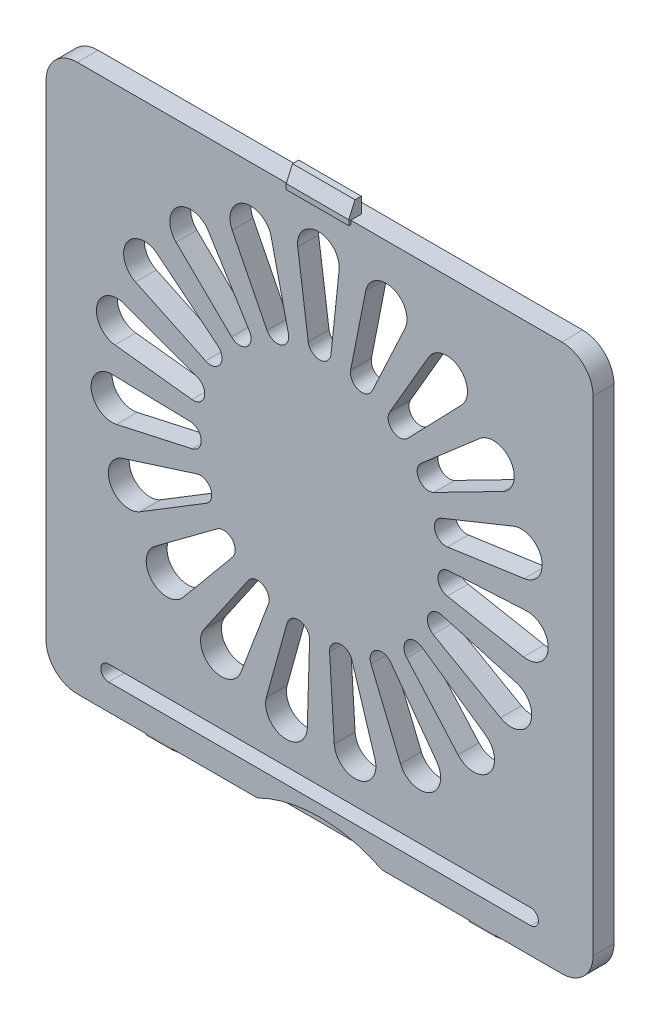
SolidWorks part; units mm, degrees
ref_plane "Front Plane" through (0, 0, 0) normal (0, 0, 1) x (1, 0, 0)
ref_plane "Top Plane" through (0, 0, 0) normal (0, 1, 0) x (1, 0, 0)
ref_plane "Right Plane" through (0, 0, 0) normal (1, 0, 0) x (0, 0, -1)
other "Configuration Table"
sketch "Sketch1" plane through (0, 0, 0) normal (0, 0, 1) x (1, 0, 0)
  line L1 (-23.25, 26.25) -> (23.25, 26.25)
  line L2 (-26.25, 23.25) -> (-26.25, -23.25)
  line L3 (-23.25, -26.25) -> (23.25, -26.25)
  line L4 (26.25, 23.25) -> (26.25, -23.25)
  line L5 (-26.25, 26.25) -> (26.25, -26.25) construction
  line L6 (-26.25, -26.25) -> (26.25, 26.25) construction
  line L11 (-20, -20) -> (20, 20) construction
  line L12 (-20, 20) -> (20, -20) construction
  arc A4 (23.25, -26.25) -> (26.25, -23.25) centre (23.25, -23.25) ccw
  arc A5 (-26.25, -23.25) -> (-23.25, -26.25) centre (-23.25, -23.25) ccw
  arc A6 (-23.25, 26.25) -> (-26.25, 23.25) centre (-23.25, 23.25) ccw
  arc A7 (23.25, 26.25) -> (26.25, 23.25) centre (23.25, 23.25) cw
  point P0 (0, 0)
  point P6 (0, 0)
  dimension "D6" = 3
  dimension "D1" = 52.5
  dimension "D2" = 52.5
extrude "Boss-Extrude1" add sketch "Sketch1" along normal blind 2
sketch "Sketch2" plane through (0, 0, 2) normal (0, 0, 1) x (1, 0, 0)
  line L6 (-20.25, -23) -> (20.25, -23) construction
  line L7 (-20.25, -22.25) -> (20.25, -22.25)
  line L8 (-20.25, -23.75) -> (20.25, -23.75)
  line L9 (26.25, -23.25) -> (26.25, 23.25) construction
  line L10 (-26.25, 23.25) -> (-26.25, -23.25) construction
  line L11 (-23.25, -26.25) -> (23.25, -26.25) construction
  line L12 (-2.0944, 21.4802) -> (-1.0899, 14.1016)
  line L13 (1.8762, 21.5399) -> (1.0939, 14.1344)
  line L14 (23.25, 26.25) -> (-23.25, 26.25) construction
  line L15 (4.4254, 21.0912) -> (2.9797, 13.7863)
  line L16 (8.2003, 19.8584) -> (5.0559, 13.1082)
  line L17 (10.4657, 18.6063) -> (6.7264, 12.1666)
  line L18 (13.6358, 16.2146) -> (8.4699, 10.8512)
  line L19 (15.3719, 14.2948) -> (9.7442, 9.4182)
  line L20 (17.5936, 11.0033) -> (10.9662, 7.6079)
  line L21 (18.6123, 8.6238) -> (11.7061, 5.8387)
  line L22 (19.6449, 4.7893) -> (12.274, 3.7298)
  line L23 (19.8358, 2.208) -> (12.3994, 1.8162)
  line L24 (19.5674, -1.754) -> (12.2518, -0.3629)
  line L25 (18.9097, -4.2575) -> (11.7491, -2.2134)
  line L26 (17.3694, -7.9177) -> (10.9019, -4.2265)
  line L27 (15.9345, -10.072) -> (9.8256, -5.8136)
  line L28 (13.2892, -13.0337) -> (8.3706, -7.4426)
  line L29 (11.2326, -14.6054) -> (6.8373, -8.5942)
  line L30 (7.7689, -16.5477) -> (4.9323, -9.6624)
  line L31 (5.3134, -17.3664) -> (3.1081, -10.2538)
  line L32 (1.4067, -18.0788) -> (0.9594, -10.6456)
  line L33 (-1.1816, -18.0559) -> (-0.9579, -10.6126)
  line L34 (-5.1079, -17.4612) -> (-3.1174, -10.2855)
  line L35 (-7.5485, -16.5991) -> (-4.9201, -9.6317)
  line L36 (-11.069, -14.7617) -> (-6.8564, -8.6211)
  line L37 (-13.0975, -13.1538) -> (-8.3492, -7.4174)
  line L38 (-15.8306, -10.273) -> (-9.8524, -5.8329)
  line L39 (-17.2271, -8.0936) -> (-10.8735, -4.2097)
  line L40 (-18.8767, -4.4813) -> (-11.7808, -2.223)
  line L41 (-19.4899, -1.9666) -> (-12.2194, -0.3562)
  line L42 (-19.8772, 1.9856) -> (-12.4325, 1.8175)
  line L43 (-19.6406, 4.5631) -> (-12.2412, 3.7255)
  line L44 (-18.7237, 8.4269) -> (-11.7369, 5.8506)
  line L45 (-17.663, 10.788) -> (-10.9365, 7.5932)
  line L46 (-15.5412, 14.1447) -> (-9.7695, 9.4394)
  line L47 (-13.7714, 16.0335) -> (-8.4466, 10.8277)
  line L48 (-10.6746, 18.5194) -> (-6.7434, 12.195)
  line L57 (-8.3873, 19.7311) -> (-5.0415, 13.0785)
  line L58 (-4.6512, 21.0768) -> (-2.9866, 13.8186)
  arc A6 (-20.25, -22.25) -> (-20.25, -23.75) centre (-20.25, -23) ccw
  arc A7 (20.25, -23.75) -> (20.25, -22.25) centre (20.25, -23) ccw
  circle A8 centre (0, 1.75) radius 12.5 construction
  arc A9 (-1.0899, 14.1016) -> (1.0939, 14.1344) centre (0, 14.25) ccw
  arc A10 (1.8762, 21.5399) -> (-2.0944, 21.4802) centre (-0.1127, 21.75) ccw
  arc A11 (8.2003, 19.8584) -> (4.4254, 21.0912) centre (6.3874, 20.7029) ccw
  arc A12 (2.9797, 13.7863) -> (5.0559, 13.1082) centre (4.0587, 13.5727) ccw
  arc A13 (13.6358, 16.2146) -> (10.4657, 18.6063) centre (12.1953, 17.602) ccw
  arc A14 (6.7264, 12.1666) -> (8.4699, 10.8512) centre (7.6777, 11.6143) ccw
  arc A15 (17.5936, 11.0033) -> (15.3719, 14.2948) centre (16.6817, 12.7833) ccw
  arc A16 (9.7442, 9.4182) -> (10.9662, 7.6079) centre (10.4646, 8.5869) ccw
  arc A17 (19.6449, 4.7893) -> (18.6123, 8.6238) centre (19.3603, 6.769) ccw
  arc A18 (11.7061, 5.8387) -> (12.274, 3.7298) centre (12.1175, 4.8186) ccw
  arc A19 (19.5674, -1.754) -> (19.8358, 2.208) centre (19.941, 0.2107) ccw
  arc A20 (12.3994, 1.8162) -> (12.2518, -0.3629) centre (12.4573, 0.7178) ccw
  arc A21 (17.3694, -7.9177) -> (18.9097, -4.2575) centre (18.3607, -6.1807) ccw
  arc A22 (11.7491, -2.2134) -> (10.9019, -4.2265) centre (11.4472, -3.2712) ccw
  arc A23 (13.2892, -13.0337) -> (15.9345, -10.072) centre (14.7908, -11.7127) ccw
  arc A24 (9.8256, -5.8136) -> (8.3706, -7.4426) centre (9.1965, -6.716) ccw
  arc A25 (7.7689, -16.5477) -> (11.2326, -14.6054) centre (9.6181, -15.7858) ccw
  arc A26 (6.8373, -8.5942) -> (4.9323, -9.6624) centre (5.9493, -9.2434) ccw
  arc A27 (1.4067, -18.0788) -> (5.3134, -17.3664) centre (3.4031, -17.9587) ccw
  arc A28 (3.1081, -10.2538) -> (0.9594, -10.6456) centre (2.0574, -10.5795) ccw
  arc A29 (-5.1079, -17.4612) -> (-1.1816, -18.0559) centre (-3.1807, -17.9958) ccw
  arc A30 (-0.9579, -10.6126) -> (-3.1174, -10.2855) centre (-2.0574, -10.5795) ccw
  arc A31 (-11.069, -14.7617) -> (-7.5485, -16.5991) centre (-9.4198, -15.8931) ccw
  arc A32 (-4.9201, -9.6317) -> (-6.8564, -8.6211) centre (-5.9493, -9.2434) ccw
  arc A33 (-15.8306, -10.273) -> (-13.0975, -13.1538) centre (-14.6381, -11.8786) ccw
  arc A34 (-8.3492, -7.4174) -> (-9.8524, -5.8329) centre (-9.1965, -6.716) ccw
  arc A35 (-18.8767, -4.4813) -> (-17.2271, -8.0936) centre (-18.2702, -6.3871) ccw
  arc A36 (-10.8735, -4.2097) -> (-11.7808, -2.223) centre (-11.4472, -3.2712) ccw
  arc A37 (-19.8772, 1.9856) -> (-19.4899, -1.9666) centre (-19.9224, -0.0139) ccw
  arc A38 (-12.2194, -0.3562) -> (-12.4325, 1.8175) centre (-12.4573, 0.7178) ccw
  arc A39 (-18.7237, 8.4269) -> (-19.6406, 4.5631) centre (-19.4157, 6.5504) ccw
  arc A40 (-12.2412, 3.7255) -> (-11.7369, 5.8506) centre (-12.1175, 4.8186) ccw
  arc A41 (-15.5412, 14.1447) -> (-17.663, 10.788) centre (-16.805, 12.5946) ccw
  arc A42 (-10.9365, 7.5932) -> (-9.7695, 9.4394) centre (-10.4646, 8.5869) ccw
  arc A43 (-10.6746, 18.5194) -> (-13.7714, 16.0335) centre (-12.3732, 17.4636) ccw
  arc A44 (-8.4466, 10.8277) -> (-6.7434, 12.195) centre (-7.6777, 11.6143) ccw
  arc A53 (-4.6512, 21.0768) -> (-8.3873, 19.7311) centre (-6.6006, 20.6297) ccw
  arc A54 (-5.0415, 13.0785) -> (-2.9866, 13.8186) centre (-4.0587, 13.5727) ccw
  point P5 (0, -23)
  dimension "D4" = 6
  dimension "D5" = 6
  dimension "D8" = 24.5
  dimension "D9" = 4.5
  dimension "D1" = 25
  dimension "D2" = 2.2
  dimension "D3" = 4
  dimension "D6" = 1.5
  dimension "D7" = 2.5
  dimension "D10" = 19
extrude "Cut-Extrude1" cut sketch "Sketch2" against normal blind 12
sketch "Sketch3" plane through (0, 0, 0) normal (0, 0, -1) x (-1, 0, 0)
  circle A0 centre (0, -38.353) radius 13.5
  dimension "D1" = 27
extrude "Cut-Extrude2" cut sketch "Sketch3" against normal blind 1 from offset 1 offset against normal yes
sketch "Sketch4" plane through (0, 0, 0) normal (1, 0, 0) x (0, 0, -1)
  line L0 (-1, -26.25) -> (-1, -27)
  line L1 (-2, -26.25) -> (0, -26.25) construction
  line L3 (-1.8923, -26.45) -> (-1.8923, -26.25)
  line L4 (-1.8923, -26.25) -> (-1, -26.25)
  line L5 (-1, -27) -> (-1.25, -27)
  line L6 (-1.25, -27) -> (-1.8923, -26.45)
  dimension "D1" = 0.75
  dimension "D2" = 0.2
  dimension "D3" = 0.25
extrude "Boss-Extrude2" add sketch "Sketch4" along normal blind 2.5 from offset 14.25
mirror "Mirror3" about plane through (0, 0, 0) normal (1, 0, 0) of "Boss-Extrude2"
sketch "Sketch5" plane through (0, 0, 0) normal (1, 0, 0) x (0, 0, -1)
  line L0 (-1, 26.25) -> (-1, 27.75)
  line L1 (-2, 26.25) -> (0, 26.25) construction
  line L2 (-1, 27.75) -> (-1.6, 27.75)
  line L3 (-1.6, 27.75) -> (-2.2, 26.392)
  line L4 (-2.2, 26.392) -> (-2.2, 25.892)
  line L5 (-2.2, 25.892) -> (-1, 25.892)
  line L6 (-1, 25.892) -> (-1, 26.25)
  line L7 (-2, 26.25) -> (-2, 23.25) construction
  dimension "D1" = 1.5
  dimension "D2" = 0.6
  dimension "D3" = 0.5
  dimension "D4" = 0.2
extrude "Boss-Extrude3" add sketch "Sketch5" along normal mid plane 6
